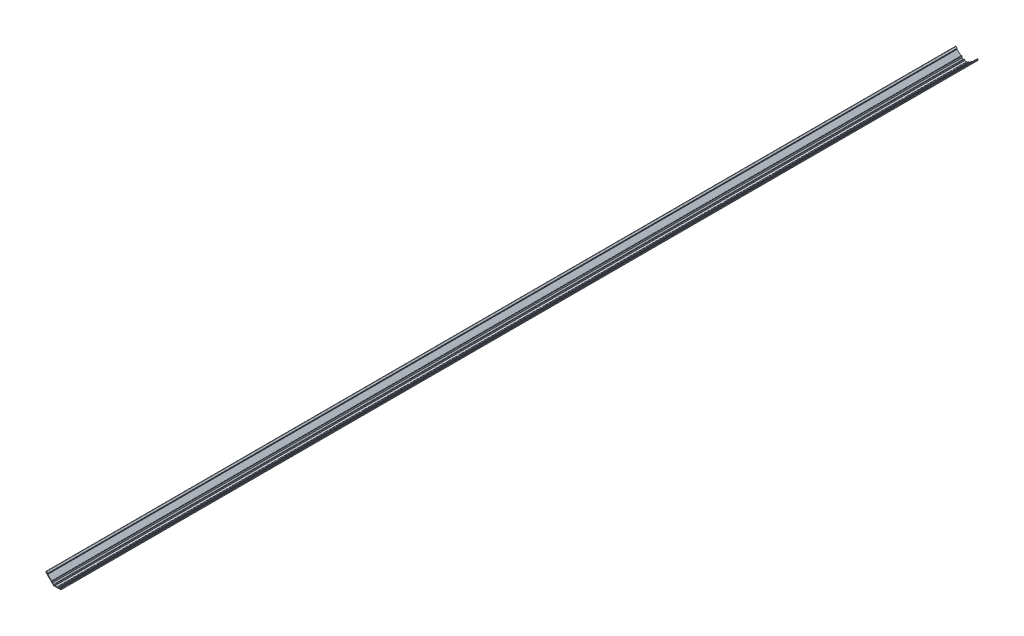
from build123d import *

# Parameters (mm, degrees)
EXTRUDE_1_DEPTH = 1142.5


with BuildPart() as part:
    # 草图2 → 凸台-拉伸1 (new, symmetric)
    with BuildSketch(Plane.XY):
        with BuildLine():
            Line((6.75, 5), (5.25, 5))
            Line((5.25, 5), (5.25, 2))
            Line((5.25, 2), (0.25, 2))
            ThreePointArc((0.25, 2), (0, 1.75), (-0.25, 2))
            Line((-0.25, 2), (-5.25, 2))
            Line((-5.25, 2), (-5.25, 5))
            Line((-5.25, 5), (-6.75, 5))
            Line((-6.75, 5), (-6.75, 2))
            Line((-6.75, 2), (-8.634653896, 2))
            Line((-8.634653896, 2), (-11.75, 5.119363474))
            Line((-11.75, 5.119363474), (-11.75, 8.88650173))
            Line((-11.75, 8.88650173), (-12.25, 9.38650173))
            Line((-12.25, 9.38650173), (-12.75, 9.38650173))
            Line((-12.75, 9.38650173), (-12.75, 7.328070483))
            ThreePointArc((-12.75, 7.328070483), (-13.058886266, 6.866036349), (-13.603902163, 6.97486621))
            Line((-13.603902163, 6.97486621), (-23.891097866, 17.282388203))
            Line((-23.891097866, 17.282388203), (-23.891097866, 19.37637924))
            Line((-23.891097866, 19.37637924), (-26.873078382, 22.358359756))
            Line((-26.873078382, 22.358359756), (-27.580185163, 22.358359756))
            Line((-27.580185163, 22.358359756), (-28.284271248, 21.654273671))
            Line((-28.284271248, 21.654273671), (-28.284271248, 19.102647866))
            Line((-28.284271248, 19.102647866), (-9.181623382, 0))
            Line((-9.181623382, 0), (9.181623382, 0))
            Line((9.181623382, 0), (28.287291944, 19.105668562))
            Line((28.287291944, 19.105668562), (28.287291944, 21.651252975))
            Line((28.287291944, 21.651252975), (27.580185163, 22.358359756))
            Line((27.580185163, 22.358359756), (26.873078382, 22.358359756))
            Line((26.873078382, 22.358359756), (23.891097866, 19.376379241))
            Line((23.891097866, 19.376379241), (23.891097866, 17.282388203))
            Line((23.891097866, 17.282388203), (13.603902163, 6.97486621))
            ThreePointArc((13.603902163, 6.97486621), (13.058886266, 6.866036349), (12.75, 7.328070483))
            Line((12.75, 7.328070483), (12.75, 9.38650173))
            Line((12.75, 9.38650173), (12.25, 9.38650173))
            Line((12.25, 9.38650173), (11.75, 8.88650173))
            Line((11.75, 8.88650173), (11.75, 5.118657708))
            Line((11.75, 5.118657708), (8.636038969, 2))
            Line((8.636038969, 2), (6.75, 2))
            Line((6.75, 2), (6.75, 5))
        make_face()
    extrude(amount=EXTRUDE_1_DEPTH, both=True)


solid = part.part
